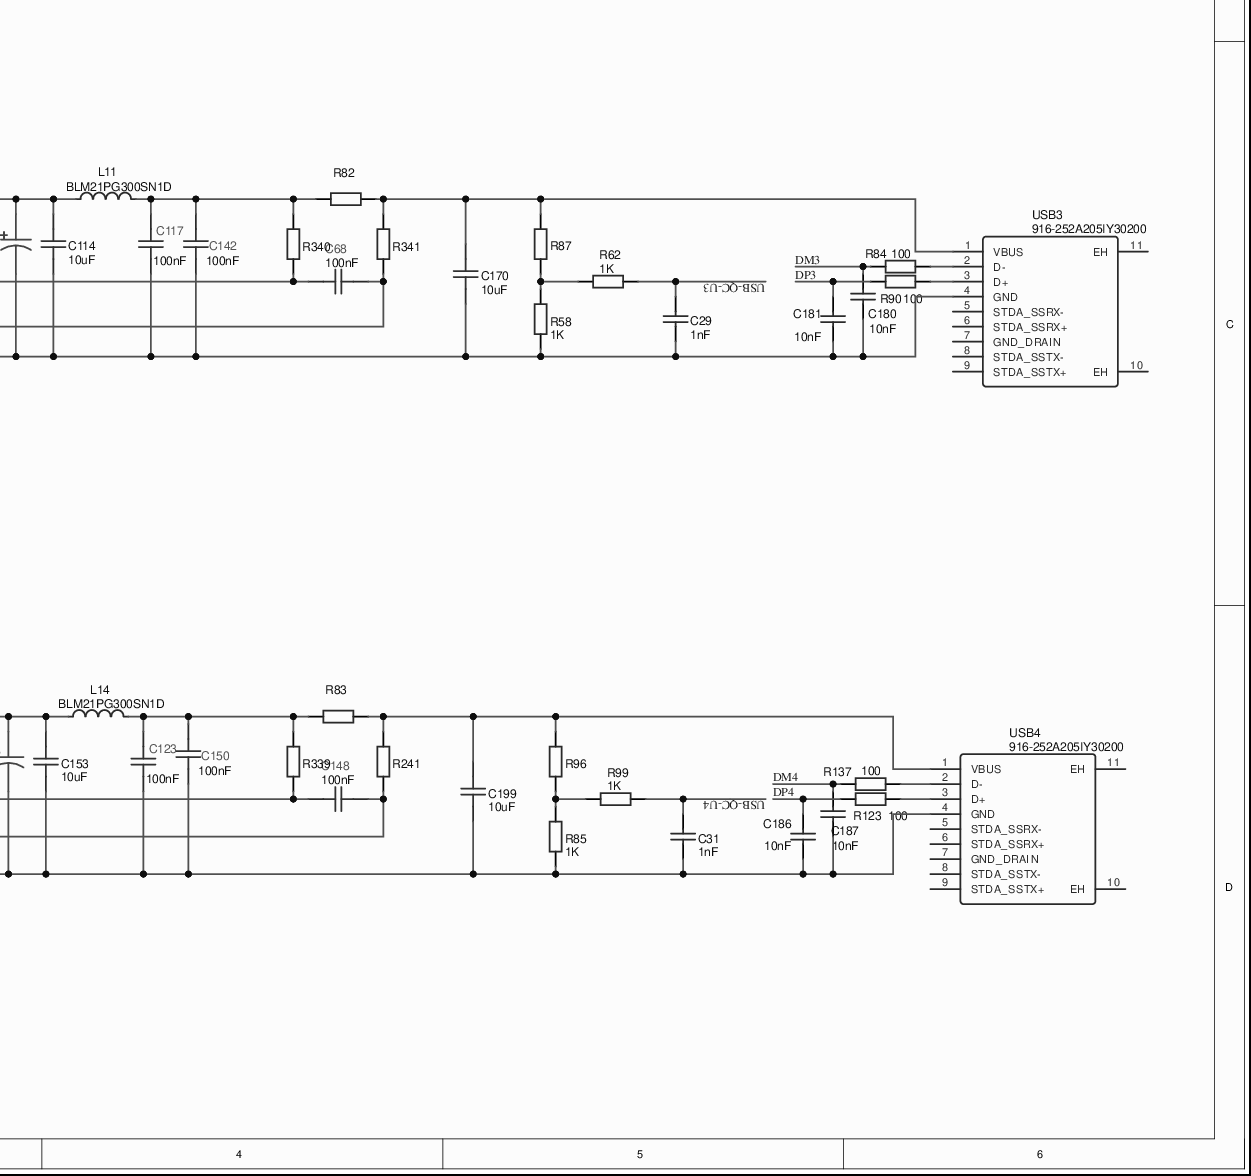
[diagram p0: MISC84402-6.SchDoc, bottom right]
# Altium project MISC84402-4.PrjPcb (part 7 of 7)

## Nets that join several sheets
GND: MISC84402-8 (29 pins), MISC84402-7 (80 pins), MISC84402-10 (22 pins), MISC84402-9 (10 pins), MISC84402-11 (20 pins), MISC84402-12 (62 pins), MISC84402-5 (62 pins), MISC84402-6 (C61.1 R59.1)
13.6V-I: MISC84402-7 (R317.2), MISC84402-12 (C43.2 D12.1 R147.2)
13.6V-U: MISC84402-7 (R86.2), MISC84402-12 (C159.1 D41.1 R295.1)
+5V: MISC84402-7 (7 pins), MISC84402-11 (C28.1 C30.1 U7.3), MISC84402-12 (Q4.2 Q45.2 R291.1 R314.1)
+12V: MISC84402-8 (10 pins), MISC84402-7 (9 pins), MISC84402-11 (C65.1 C96.1 U16.3), MISC84402-12 (R48.2 R362.1)
+13.6V: MISC84402-8 (F2.1 F3.1 F4.1), MISC84402-12 (10 pins)
+13.6V-F: MISC84402-8 (CON1.1 R197.1), MISC84402-12 (7 pins)
+24V: MISC84402-12 (6 pins), MISC84402-5 (16 pins), MISC84402-6 (16 pins)
+VCC_BAT: MISC84402-11 (6 pins), MISC84402-12 (C44.1 C54.1 U2.8)
B+: MISC84402-11 (F6.1), MISC84402-12 (10 pins)
BMS_EN: MISC84402-10 (CN1.4), MISC84402-11 (KEY6.1 KEY6.2)
BUSY: MISC84402-7 (U13.90), MISC84402-9 (C168.2 R321.1 R322.2)
Car-EN: MISC84402-8 (R191.1), MISC84402-7 (U13.59)
Car-I: MISC84402-8 (C51.2 R67.2), MISC84402-7 (R356.2)
DC1-EN: MISC84402-8 (R32.1), MISC84402-7 (U13.58)
DC1-I: MISC84402-8 (C53.2 R69.2), MISC84402-7 (R354.2)
DC2-EN: MISC84402-8 (R40.1), MISC84402-7 (U13.57)
DC2-I: MISC84402-8 (C56.2 R70.2), MISC84402-7 (R355.2)
EN9V-INT: MISC84402-7 (U13.61), MISC84402-10 (C2.2 D11.1 R270.2)
EN_485_INV: MISC84402-7 (U13.70), MISC84402-10 (R176.1)
EN_BMS_IN: MISC84402-7 (U13.77), MISC84402-10 (R184.1)
EN_INV: MISC84402-7 (U13.64), MISC84402-10 (CN3.4)
FAN1: MISC84402-8 (C93.2 D57.1 R276.2 R298.2), MISC84402-7 (U13.18)
FAN1-EN: MISC84402-8 (R186.1), MISC84402-7 (U13.95)
LED-EN: MISC84402-8 (R287.1), MISC84402-7 (U13.88)
PC UART-RX: MISC84402-7 (R47.1), MISC84402-5 (USB1.B8)
PC UART-TX: MISC84402-7 (R324.1), MISC84402-5 (USB1.A8)
POW13.6-EN: MISC84402-7 (U13.82), MISC84402-12 (R73.1)
POW24-EN: MISC84402-7 (U13.81), MISC84402-12 (R302.1)
RX_485_INV: MISC84402-7 (U13.69), MISC84402-10 (D27.2 R158.2)
RX_BMS_IN: MISC84402-7 (U13.79), MISC84402-10 (D26.2 R38.2)
RXD-MODBUS: MISC84402-7 (U13.86), MISC84402-9 (R140.1)
SCK1: MISC84402-7 (R249.2 U13.51), MISC84402-5 (R127.2)
SCK2: MISC84402-7 (R94.2 U13.53), MISC84402-5 (R199.2)
SDA1: MISC84402-7 (R246.2 U13.52), MISC84402-5 (R128.2)
SDA2: MISC84402-7 (R283.2 U13.54), MISC84402-5 (R200.2)
TX_485_INV: MISC84402-7 (U13.68), MISC84402-10 (R165.1)
TX_BMS_IN: MISC84402-7 (U13.78), MISC84402-10 (R159.1)
TXD-MODBUS: MISC84402-7 (U13.87), MISC84402-9 (Q42.3 R320.1)
USB-QC-I: MISC84402-7 (R282.2), MISC84402-6 (C61.2 R77.1)
USB-QC-U1: MISC84402-7 (R280.1), MISC84402-6 (C62.2 R103.2)
USB-QC-U2: MISC84402-7 (R284.2), MISC84402-6 (C46.2 R17.2)
USB-QC-U3: MISC84402-7 (R285.1), MISC84402-6 (C29.2 R62.2)
USB-QC-U4: MISC84402-7 (R286.1), MISC84402-6 (C31.2 R99.2)
VCC9V: MISC84402-7 (C78.2 C87.1 U8.3), MISC84402-10 (CN3.6 R270.1)
VDD5V: MISC84402-7 (Q50.3), MISC84402-10 (R229.2 R231.2 R232.1 R244.1), MISC84402-9 (R144.2 R153.2 U12.1 U12.2)
VDD 3.3V: MISC84402-7 (21 pins), MISC84402-10 (6 pins), MISC84402-9 (R319.2 R320.2)